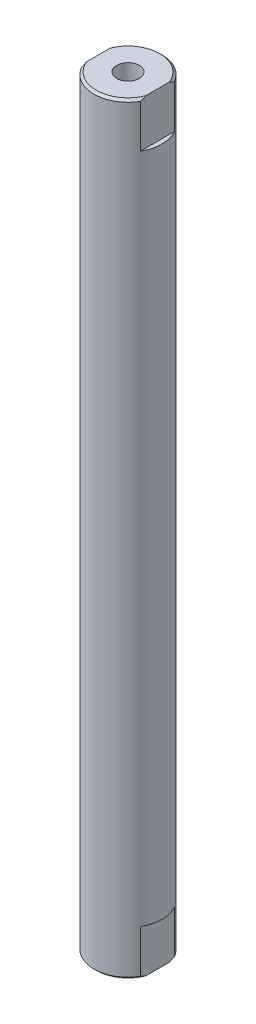
from build123d import *

# Parameters (mm, degrees)
SKETCH_1_R          = 7.5
EXTRUDE_1_DEPTH     = 84
CHAMFER_1_SIZE      = 0.5
SKETCH_4_W          = 1
SKETCH_4_H          = 10
CUT_EXTRUDE_1_DEPTH = 10


with BuildPart() as part:
    # 草图1 → 凸台-拉伸1 (new, symmetric)
    with BuildSketch(Plane(origin=(0, 0, 0), x_dir=(1, 0, 0), z_dir=(0, 1, 0))):
        with Locations(Location((0, 0, 0), (0, 0, 90))):
            Circle(SKETCH_1_R)
    extrude(amount=EXTRUDE_1_DEPTH, both=True)

    # 倒角1
    chamfer_1_edges = [part.edges().sort_by_distance(p)[0] for p in [
        (0, -84, 7.5),
        (0, 84, 7.5),
    ]]
    chamfer(chamfer_1_edges, length=CHAMFER_1_SIZE)

    # 草图2 → M6 螺纹孔1 (revolve, cut)
    with BuildSketch(Plane(origin=(0, 84, 0), x_dir=(0, 0, 1), z_dir=(1, 0, 0))):
        Polygon((0, 0), (0, 18.502151548), (2.5, 17), (2.5, 0), align=None)
    hole_wizard_m6_1 = revolve(axis=Axis((0, 90.35, 0), (0, -1, 0)), mode=Mode.SUBTRACT)

    # 镜向1: M6 螺纹孔1 across plane
    add(hole_wizard_m6_1.mirror(Plane.ZX), mode=Mode.SUBTRACT)

    # 草图4 → 切除-拉伸1 (cut, symmetric)
    with BuildSketch(Plane.XY):
        with Locations((-7, 79)):
            Rectangle(SKETCH_4_W, SKETCH_4_H)
        with Locations((7, 79)):
            Rectangle(SKETCH_4_W, SKETCH_4_H)
        with Locations((7, -79)):
            Rectangle(SKETCH_4_W, SKETCH_4_H)
        with Locations((-7, -79)):
            Rectangle(SKETCH_4_W, SKETCH_4_H)
    extrude(amount=CUT_EXTRUDE_1_DEPTH, both=True, mode=Mode.SUBTRACT)


solid = part.part
